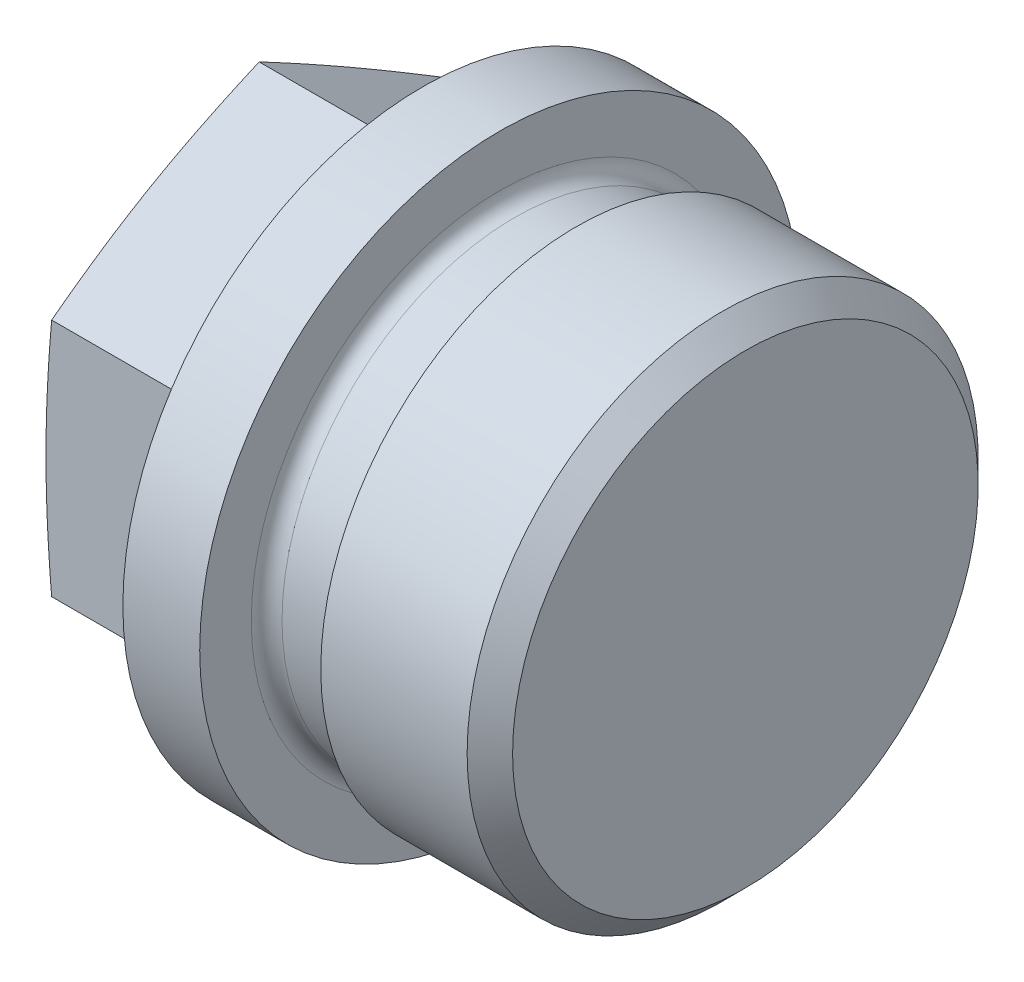
from build123d import *

# Parameters (mm, degrees)
EXTRUDE1_DEPTH     = 11
SKETCH3_OUTSIDE_W  = 167.178
SKETCH3_OUTSIDE_H  = 167.178
SKETCH3_OUTSIDE_R  = 13.5
CUT_EXTRUDE1_DEPTH = 10
CUT_EXTRUDE1_DRAFT = -80
FILLET1_R          = 1


with BuildPart() as part:
    # Sketch1 → Revolve1 (revolve)
    with BuildSketch(Plane.XY, mode=Mode.PRIVATE) as revolve1_sk:
        Polygon((21, 16.6245), (21, 15.1455), (16, 15.1455), (16, 19.5), (11, 19.5), (11, 1.5), (0, 1.5), (0, 0), (32, 0), (32, 15.1455), (30.521, 16.6245), align=None)
    revolve(revolve1_sk.sketch.rotate(Axis((0, 0, 0), (1, 0, 0)), 90), axis=Axis((0, 0, 0), (1, 0, 0)))

    # Sketch2 → Extrude1 (add)
    with BuildSketch(Plane.ZY):
        Polygon((0, 15.588457268), (-13.5, 7.794228634), (-13.5, -7.794228634), (0, -15.588457268), (13.5, -7.794228634), (13.5, 7.794228634), align=None)
    extrude(amount=-EXTRUDE1_DEPTH)


with BuildPart() as cut_extrude1_tool:
    # Sketch3 outside → Cut-Extrude1 (with draft: the straight prism first)
    with BuildSketch(Plane.ZY):
        Rectangle(SKETCH3_OUTSIDE_W, SKETCH3_OUTSIDE_H)
        Circle(SKETCH3_OUTSIDE_R, mode=Mode.SUBTRACT)
    extrude(amount=-CUT_EXTRUDE1_DEPTH)
    # Cut-Extrude1: the draft: its side faces are tilted about the plane it starts from
    cut_extrude1_sides = [cut_extrude1_tool.faces().sort_by_distance(p)[0] for p in [
        (5, -83.589, 0),
        (5, 0, 83.589),
        (5, 83.589, 0),
        (5, 0, -83.589),
        (5, 0, -13.5),
    ]]
    draft(cut_extrude1_sides, Plane.ZY, CUT_EXTRUDE1_DRAFT)


with BuildPart() as part_1:
    add(part.part)

    # Cut-Extrude1: cut by cut_extrude1_tool
    add(cut_extrude1_tool.part, mode=Mode.SUBTRACT)

    # Fillet1
    fillet1_edges = [part_1.edges().sort_by_distance(p)[0] for p in [
        (21, 0, -15.1455),
        (16, 0, -15.1455),
    ]]
    fillet(fillet1_edges, radius=FILLET1_R)


solid = part_1.part
